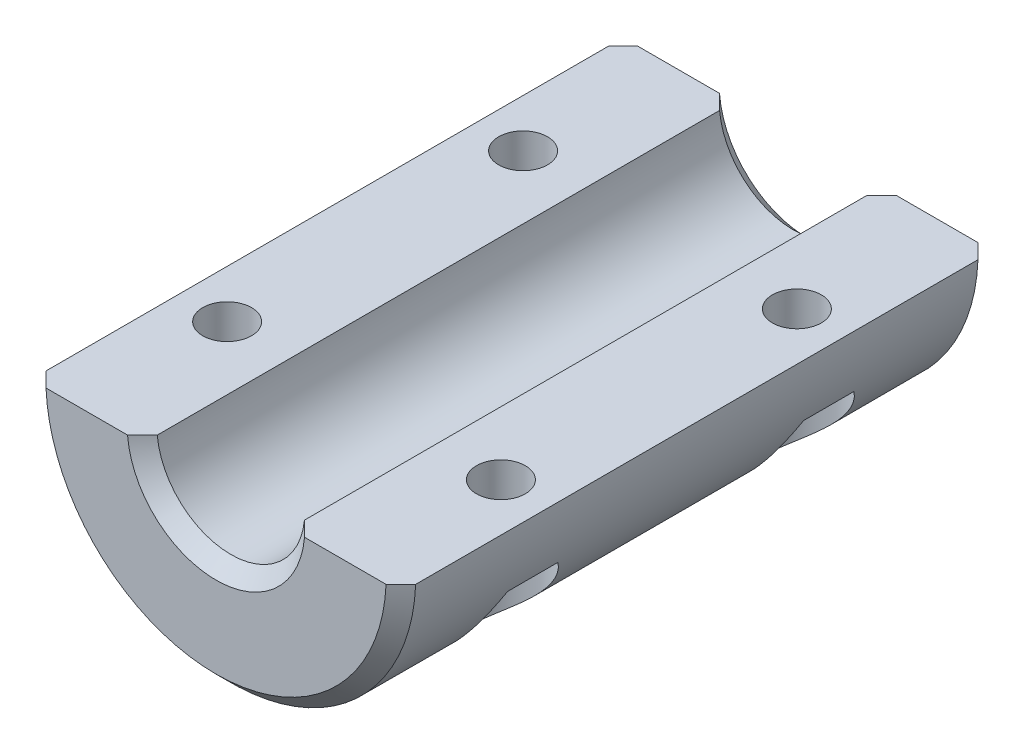
from build123d import *

# Parameters (mm, degrees)
EXTRUDE_1_DEPTH           = 80
SKETCH_2_R                = 5.5
CUT_EXTRUDE_1_DEPTH       = 100
HOLE_WIZARD_1_D           = 6.6
HOLE_WIZARD_1_CBORE_D     = 11
HOLE_WIZARD_1_CBORE_DEPTH = 6.8
CHAMFER_1_SIZE            = 2


with BuildPart() as part:
    # 草图1 → 凸台-拉伸1 (new body)
    with BuildSketch(Plane.XY):
        with BuildLine():
            Line((-24.979991994, -1), (-9.949874371, -1))
            ThreePointArc((-9.949874371, -1), (0, -10), (9.949874371, -1))
            Line((9.949874371, -1), (24.979991994, -1))
            ThreePointArc((24.979991994, -1), (0, -25), (-24.979991994, -1))
        make_face()
    extrude(amount=EXTRUDE_1_DEPTH)

    # 草图2 → 切除-拉伸1 (cut)
    with BuildSketch(Plane(origin=(0, -17, 0), x_dir=(1, 0, 0), z_dir=(0, 1, 0))):
        with Locations((-18.5, -20)):
            Circle(SKETCH_2_R)
        with Locations((18.5, -20)):
            Circle(SKETCH_2_R)
        with Locations((18.5, -60)):
            Circle(SKETCH_2_R)
        with Locations((-18.5, -60)):
            Circle(SKETCH_2_R)
    extrude(amount=-CUT_EXTRUDE_1_DEPTH, mode=Mode.SUBTRACT)

    # 打孔尺寸(%根据)内六角圆柱头螺钉的类型1 (through all)
    with Locations(Plane(origin=(0, -17, 0), x_dir=(-1, 0, 0), z_dir=(0, -1, 0))):
        with Locations((-18.5, -20), (18.5, -20), (18.5, -60), (-18.5, -60)):
            CounterBoreHole(HOLE_WIZARD_1_D / 2, HOLE_WIZARD_1_CBORE_D / 2, HOLE_WIZARD_1_CBORE_DEPTH)

    # 倒角1
    chamfer_1_edges = [part.edges().sort_by_distance(p)[0] for p in [
        (0, -25, 80),
        (0, -10, 80),
        (0, -25, 0),
        (0, -10, 0),
    ]]
    chamfer(chamfer_1_edges, length=CHAMFER_1_SIZE)


solid = part.part
